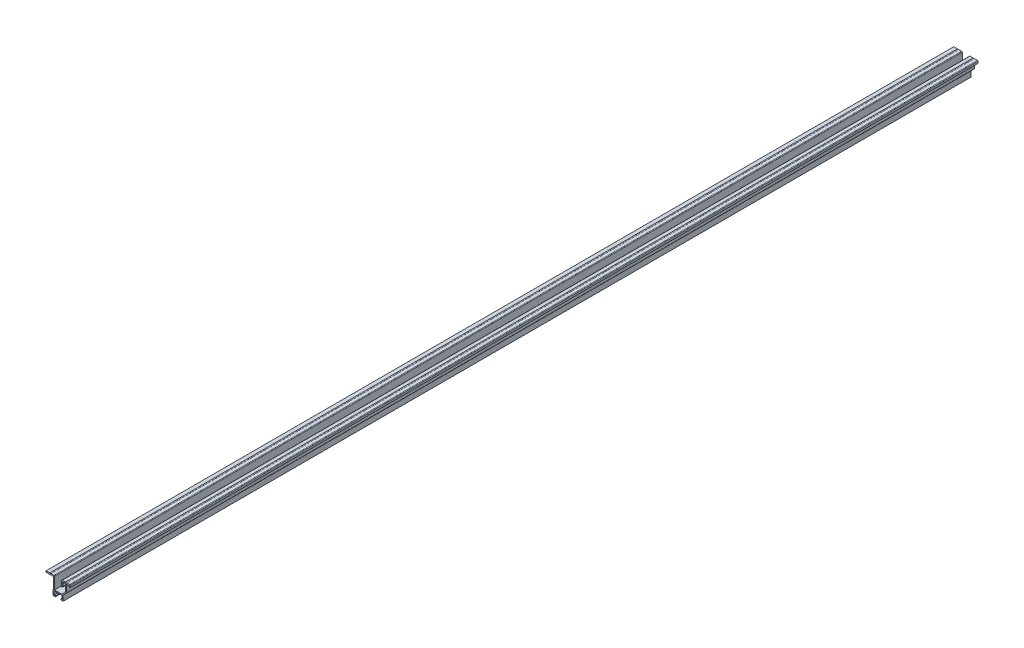
from build123d import *

# Parameters (mm, degrees)
EXTRUDE_1_DEPTH     = 750
CUT_EXTRUDE_1_DEPTH = 752.345626193


with BuildPart() as part:
    # 草图1 → 凸台-拉伸1 (new, symmetric)
    with BuildSketch(Plane.XY):
        with BuildLine():
            Line((11.75, -20.5), (12.5, -20.5))
            Line((12.5, -20.5), (12.5, -3))
            ThreePointArc((12.5, -3), (12.207106781, -2.292893219), (11.5, -2))
            Line((11.5, -2), (0, -2))
            Line((0, -2), (0, 0))
            Line((0, 0), (6.1, 0))
            ThreePointArc((6.1, 0), (7, -0.3), (7.9, 0))
            Line((7.9, 0), (13, 0))
            ThreePointArc((13, 0), (13.707106781, -0.292893219), (14, -1))
            Line((14, -1), (14, -20.5))
            Line((14, -20.5), (26.170393622, -20.5))
            Line((26.170393622, -20.5), (32.5, -13.908507718))
            Line((32.5, -13.908507718), (32.5, -7))
            Line((32.5, -7), (27.5, -7))
            Line((27.5, -7), (27, -10))
            Line((27, -10), (26, -10))
            Line((26, -10), (26, -1))
            ThreePointArc((26, -1), (26.292893219, -0.292893219), (27, 0))
            Line((27, 0), (32.1, 0))
            ThreePointArc((32.1, 0), (33, -0.3), (33.9, 0))
            Line((33.9, 0), (39, 0))
            ThreePointArc((39, 0), (39.707106781, -0.292893219), (40, -1))
            Line((40, -1), (40, -4))
            Line((40, -4), (38, -4))
            Line((38, -4), (38, -2))
            Line((38, -2), (34, -2))
            Line((34, -2), (34, -14.512095167))
            Line((34, -14.512095167), (28.25, -20.5))
            Line((28.25, -20.5), (28.25, -29.5))
            Line((28.25, -29.5), (24.5, -29.5))
            Line((24.5, -29.5), (24.5, -28))
            Line((24.5, -28), (26.75, -28))
            Line((26.75, -28), (26.75, -22))
            Line((26.75, -22), (13.25, -22))
            Line((13.25, -22), (13.25, -28))
            Line((13.25, -28), (15.5, -28))
            Line((15.5, -28), (15.5, -29.5))
            Line((15.5, -29.5), (11.75, -29.5))
            Line((11.75, -29.5), (11.75, -20.5))
        make_face()
        with BuildLine():
            Line((32.5, -2), (32.5, -5.5))
            Line((32.5, -5.5), (27.5, -5.5))
            Line((27.5, -5.5), (27.5, -3))
            ThreePointArc((27.5, -3), (27.792893219, -2.292893219), (28.5, -2))
            Line((28.5, -2), (32.5, -2))
        make_face(mode=Mode.SUBTRACT)
    extrude(amount=EXTRUDE_1_DEPTH, both=True)

    # 草图2 → 切除-拉伸1 (cut, through all)
    with BuildSketch(Plane(origin=(0, -20.5, 0), x_dir=(1, 0, 0), z_dir=(0, 1, 0))):
        with BuildLine():
            Line((15, -550), (15, -500))
            ThreePointArc((15, -500), (20, -495), (25, -500))
            Line((25, -500), (25, -550))
            ThreePointArc((25, -550), (20, -555), (15, -550))
        make_face()
        with BuildLine():
            Line((15, 550), (15, 500))
            ThreePointArc((15, 500), (20, 495), (25, 500))
            Line((25, 500), (25, 550))
            ThreePointArc((25, 550), (20, 555), (15, 550))
        make_face()
    extrude(amount=-CUT_EXTRUDE_1_DEPTH, mode=Mode.SUBTRACT)


solid = part.part
